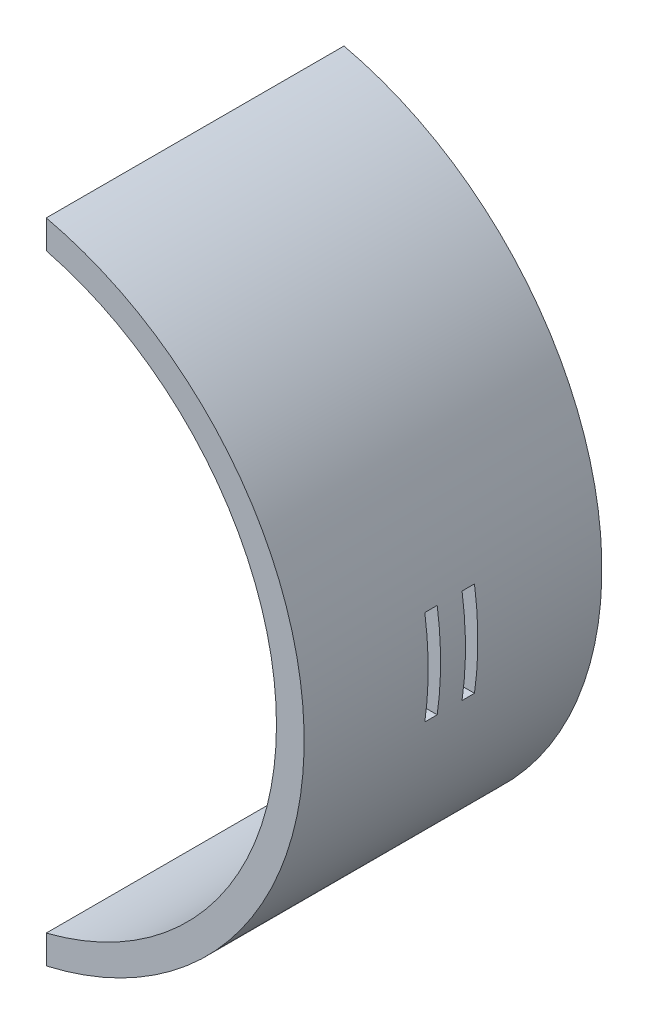
SolidWorks part; units mm, degrees
ref_plane "前视基准面" through (0, 0, 0) normal (0, 0, 1) x (1, 0, 0)
ref_plane "上视基准面" through (0, 0, 0) normal (0, 1, 0) x (1, 0, 0)
ref_plane "右视基准面" through (0, 0, 0) normal (1, 0, 0) x (0, 0, -1)
other "Configuration Table"
sketch "草图1" plane through (0, 0, 0) normal (0, 0, 1) x (1, 0, 0)
  line L0 (0, 75.5869) -> (0, -82.9026) construction
  line L1 (-115.0732, 0) -> (127.6748, 0) construction
  line L2 (15, 70.8031) -> (15, -74.287) construction
  line L3 (15, 65.2763) -> (15, 59.5355)
  line L4 (15, -59.5355) -> (15, -65.2763)
  arc A0 (15, -65.2763) -> (15, 65.2763) centre (0, 0) ccw
  arc A1 (15, -59.5355) -> (15, 59.5355) centre (0, 0) ccw
  dimension "D1" = 15
extrude "凸台-拉伸1" add sketch "草图1" along normal blind 60
sketch "草图3" plane through (0, 0, 0) normal (1, 0, 0) x (0, 0, -1)
  line L0 (-107.73, 0) -> (68.1852, 0) construction
  line L1 (-32.5039, 69.89) -> (-32.5039, -77.1331) construction
  line L2 (-30, 73.0748) -> (-30, -80.8617) construction
  line L3 (-60, 65.2763) -> (-60, -65.2763) construction
  line L10 (-32.5039, -9.55) -> (-32.5039, 9.55)
  line L11 (-32.5039, 9.55) -> (-35.0039, 9.55)
  line L12 (-35.0039, 9.55) -> (-35.0039, -9.55)
  line L13 (-32.5039, -9.55) -> (-35.0039, -9.55)
  line L14 (-27.4961, -9.55) -> (-27.4961, 9.55)
  line L15 (-27.4961, -9.55) -> (-24.9961, -9.55)
  line L16 (-24.9961, 9.55) -> (-24.9961, -9.55)
  line L17 (-27.4961, 9.55) -> (-24.9961, 9.55)
  point P14 (-30, 5.0079)
  point P15 (-30, 7.5079)
  point P18 (-32.5039, 0)
  point P19 (-35.0039, 0)
  dimension "D1" = 2.5039
  dimension "D2" = 30
  dimension "D3" = 2.5
  dimension "D4" = 9.55
extrude "切除-拉伸2" cut sketch "草图3" along normal blind 115
